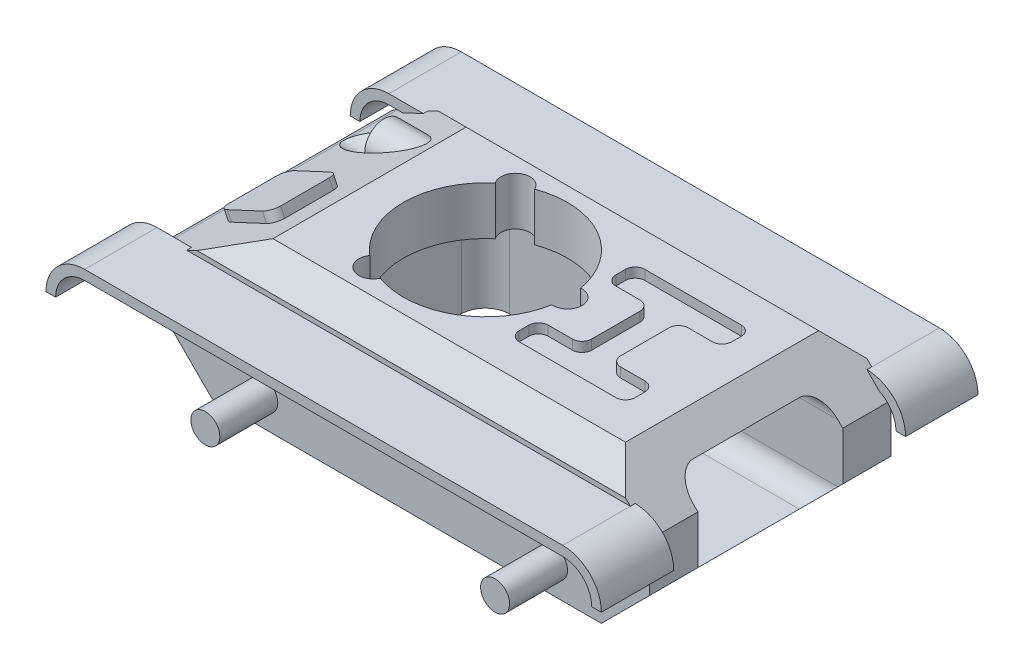
from build123d import *

# Parameters (mm, degrees)
BOSS_EXTRUDE1_DEPTH = 25
CHAMFER1_SIZE       = 5
BOSS_EXTRUDE2_DEPTH = 2
CUT_EXTRUDE1_DEPTH  = 2
CUT_EXTRUDE2_DEPTH  = 8
CUT_EXTRUDE3_DEPTH  = 38
CUT_EXTRUDE4_DEPTH  = 20
CUT_EXTRUDE6_START  = -80
SKETCH7_R           = 4
CUT_EXTRUDE6_DEPTH  = 30
BOSS_EXTRUDE3_START = -1
BOSS_EXTRUDE3_DEPTH = 15
SKETCH9_R           = 3
BOSS_EXTRUDE4_DEPTH = 12
SKETCH10_R          = 4
SKETCH10_R_2        = 3
BOSS_EXTRUDE5_DEPTH = 14


with BuildPart() as part:
    # Sketch1 → Boss-Extrude1 (new, symmetric)
    with BuildSketch(Plane.XY):
        with BuildLine():
            Line((0, 0), (-80.626570136, 0))
            Line((-80.626570136, 0), (-93.611495141, 12.984925005))
            ThreePointArc((-93.611495141, 12.984925005), (-95, 17.388699799), (-92.189052544, 21.051997846))
            Line((-92.189052544, 21.051997846), (-73, 30))
            Line((-73, 30), (0, 30))
            Line((0, 30), (10, 20))
            Line((10, 20), (10, 10))
            Line((10, 10), (0, 0))
        make_face()
    extrude(amount=BOSS_EXTRUDE1_DEPTH, both=True)

    # Chamfer1
    chamfer1_edges = [part.edges().sort_by_distance(p)[0] for p in [
        (-36.5, 30, -25),
        (-36.5, 30, 25),
    ]]
    chamfer(chamfer1_edges, length=CHAMFER1_SIZE)

    # Sketch3 → Boss-Extrude2 (add)
    with BuildSketch(Plane(origin=(-24.528918893, 52.602436319, 0), x_dir=(0.9063077870366526, 0.4226182617406939, 0), z_dir=(-0.4226182617406939, 0.9063077870366526, 0))):
        with BuildLine():
            Line((-68.481920601, -15), (-60.481920601, -15))
            ThreePointArc((-60.481920601, -15), (-59.067707039, -14.414213562), (-58.481920601, -13))
            Line((-58.481920601, -13), (-58.481920601, -3))
            ThreePointArc((-58.481920601, -3), (-59.067707039, -1.585786438), (-60.481920601, -1))
            Line((-60.481920601, -1), (-68.481920601, -1))
            ThreePointArc((-68.481920601, -1), (-69.896134164, -1.585786438), (-70.481920601, -3))
            Line((-70.481920601, -3), (-70.481920601, -13))
            ThreePointArc((-70.481920601, -13), (-69.896134164, -14.414213562), (-68.481920601, -15))
        make_face()
    extrude(amount=BOSS_EXTRUDE2_DEPTH)

    # Sketch2 → Cut-Extrude1 (cut)
    with BuildSketch(Plane(origin=(0, 30, 0), x_dir=(1, 0, 0), z_dir=(0, 1, 0))):
        with BuildLine():
            Line((-14, -7), (-9, -7))
            ThreePointArc((-9, -7), (-7.585786438, -7.585786438), (-7, -9))
            Line((-7, -9), (-7, -11))
            ThreePointArc((-7, -11), (-7.585786438, -12.414213562), (-9, -13))
            Line((-9, -13), (-29, -13))
            ThreePointArc((-29, -13), (-30.414213562, -12.414213562), (-31, -11))
            Line((-31, -11), (-31, -9))
            ThreePointArc((-31, -9), (-30.414213562, -7.585786438), (-29, -7))
            Line((-29, -7), (-24, -7))
            ThreePointArc((-24, -7), (-22.585786438, -6.414213562), (-22, -5))
            Line((-22, -5), (-22, 5))
            ThreePointArc((-22, 5), (-22.585786438, 6.414213562), (-24, 7))
            Line((-24, 7), (-29, 7))
            ThreePointArc((-29, 7), (-30.414213562, 7.585786438), (-31, 9))
            Line((-31, 9), (-31, 11))
            ThreePointArc((-31, 11), (-30.414213562, 12.414213562), (-29, 13))
            Line((-29, 13), (-9, 13))
            ThreePointArc((-9, 13), (-7.585786438, 12.414213562), (-7, 11))
            Line((-7, 11), (-7, 9))
            ThreePointArc((-7, 9), (-7.585786438, 7.585786438), (-9, 7))
            Line((-9, 7), (-14, 7))
            ThreePointArc((-14, 7), (-15.414213562, 6.414213562), (-16, 5))
            Line((-16, 5), (-16, -5))
            ThreePointArc((-16, -5), (-15.414213562, -6.414213562), (-14, -7))
        make_face()
        with BuildLine():
            ThreePointArc((-59.95558989, 12.999040356), (-66, 0), (-59.95558989, -12.999040356))
            ThreePointArc((-59.95558989, -12.999040356), (-59, -17.320508076), (-54.779704228, -15.987339336))
            ThreePointArc((-54.779704228, -15.987339336), (-40.5, -14.722431864), (-32.264705882, -2.98829898))
            ThreePointArc((-32.264705882, -2.98829898), (-29, 0), (-32.264705882, 2.98829898))
            ThreePointArc((-32.264705882, 2.98829898), (-40.5, 14.722431864), (-54.779704228, 15.987339336))
            ThreePointArc((-54.779704228, 15.987339336), (-59, 17.320508076), (-59.95558989, 12.999040356))
        make_face()
    extrude(amount=-CUT_EXTRUDE1_DEPTH, mode=Mode.SUBTRACT)

    # Sketch4 → Cut-Extrude2 (cut)
    with BuildSketch(Plane(origin=(0, 28, 0), x_dir=(1, 0, 0), z_dir=(0, 1, 0))):
        with BuildLine():
            ThreePointArc((-54.779704228, -15.987339336), (-40.5, -14.722431864), (-32.264705882, -2.98829898))
            ThreePointArc((-32.264705882, -2.98829898), (-29, 0), (-32.264705882, 2.98829898))
            ThreePointArc((-32.264705882, 2.98829898), (-40.5, 14.722431864), (-54.779704228, 15.987339336))
            ThreePointArc((-54.779704228, 15.987339336), (-59, 17.320508076), (-59.95558989, 12.999040356))
            ThreePointArc((-59.95558989, 12.999040356), (-66, 0), (-59.95558989, -12.999040356))
            ThreePointArc((-59.95558989, -12.999040356), (-59, -17.320508076), (-54.779704228, -15.987339336))
        make_face()
    extrude(amount=-CUT_EXTRUDE2_DEPTH, mode=Mode.SUBTRACT)

    # Sketch5 → Cut-Extrude3 (cut)
    with BuildSketch(Plane(origin=(10, 0, 0), x_dir=(0, 0, -1), z_dir=(1, 0, 0))):
        with BuildLine():
            Line((-11, 5), (11, 5))
            ThreePointArc((11, 5), (13.828427125, 6.171572875), (15, 9))
            Line((15, 9), (15, 21))
            ThreePointArc((15, 21), (13.828427125, 23.828427125), (11, 25))
            Line((11, 25), (-11, 25))
            ThreePointArc((-11, 25), (-13.828427125, 23.828427125), (-15, 21))
            Line((-15, 21), (-15, 9))
            ThreePointArc((-15, 9), (-13.828427125, 6.171572875), (-11, 5))
        make_face()
    extrude(amount=-CUT_EXTRUDE3_DEPTH, mode=Mode.SUBTRACT)

    # Sketch6 → Cut-Extrude4 (cut)
    with BuildSketch(Plane.XZ):
        with BuildLine():
            Line((-65, -21), (-33, -21))
            ThreePointArc((-33, -21), (-29.464466094, -19.535533906), (-28, -16))
            Line((-28, -16), (-28, 16))
            ThreePointArc((-28, 16), (-29.464466094, 19.535533906), (-33, 21))
            Line((-33, 21), (-65, 21))
            ThreePointArc((-65, 21), (-68.535533906, 19.535533906), (-70, 16))
            Line((-70, 16), (-70, -16))
            ThreePointArc((-70, -16), (-68.535533906, -19.535533906), (-65, -21))
        make_face()
    extrude(amount=-CUT_EXTRUDE4_DEPTH, mode=Mode.SUBTRACT)

    # Sketch7 → Cut-Extrude6 (cut)
    with BuildSketch(Plane(origin=(10, 0, 0), x_dir=(0, 0, -1), z_dir=(1, 0, 0)).offset(CUT_EXTRUDE6_START)):
        with Locations(Location((14, 25, 0), (0, 0, 90))):
            Circle(SKETCH7_R)
    extrude(amount=-CUT_EXTRUDE6_DEPTH, mode=Mode.SUBTRACT)

    # Sketch8 → Boss-Extrude3 (add)
    with BuildSketch(Plane.XY.offset(25).offset(BOSS_EXTRUDE3_START)):
        with BuildLine():
            Line((-93, 24), (6, 24))
            ThreePointArc((6, 24), (11.656854249, 21.656854249), (14, 16))
            Line((14, 16), (12, 16))
            ThreePointArc((12, 16), (10.242640687, 20.242640687), (6, 22))
            Line((6, 22), (-93, 22))
            ThreePointArc((-93, 22), (-97.242640687, 20.242640687), (-99, 16))
            Line((-99, 16), (-101, 16))
            ThreePointArc((-101, 16), (-98.656854249, 21.656854249), (-93, 24))
        make_face()
    boss_extrude3 = extrude(amount=BOSS_EXTRUDE3_DEPTH)

    # Sketch9 → Boss-Extrude4 (add)
    with BuildSketch(Plane.XY.offset(25)):
        with Locations((-70, 6)):
            Circle(SKETCH9_R)
        with Locations((-10, 6)):
            Circle(SKETCH9_R)
    boss_extrude4 = extrude(amount=BOSS_EXTRUDE4_DEPTH)

    # Mirror1: Boss-Extrude3, Boss-Extrude4 across plane
    add(boss_extrude3.mirror(Plane.XY))
    add(boss_extrude4.mirror(Plane.XY))

    # Sketch10 → Boss-Extrude5 (add)
    with BuildSketch(Plane.ZY.offset(70)):
        with Locations((-14, 25)):
            Circle(SKETCH10_R)
        with Locations(Location((-14, 25, 0), (0, 0, 270))):
            Circle(SKETCH10_R_2, mode=Mode.SUBTRACT)
    extrude(amount=BOSS_EXTRUDE5_DEPTH)


solid = part.part
